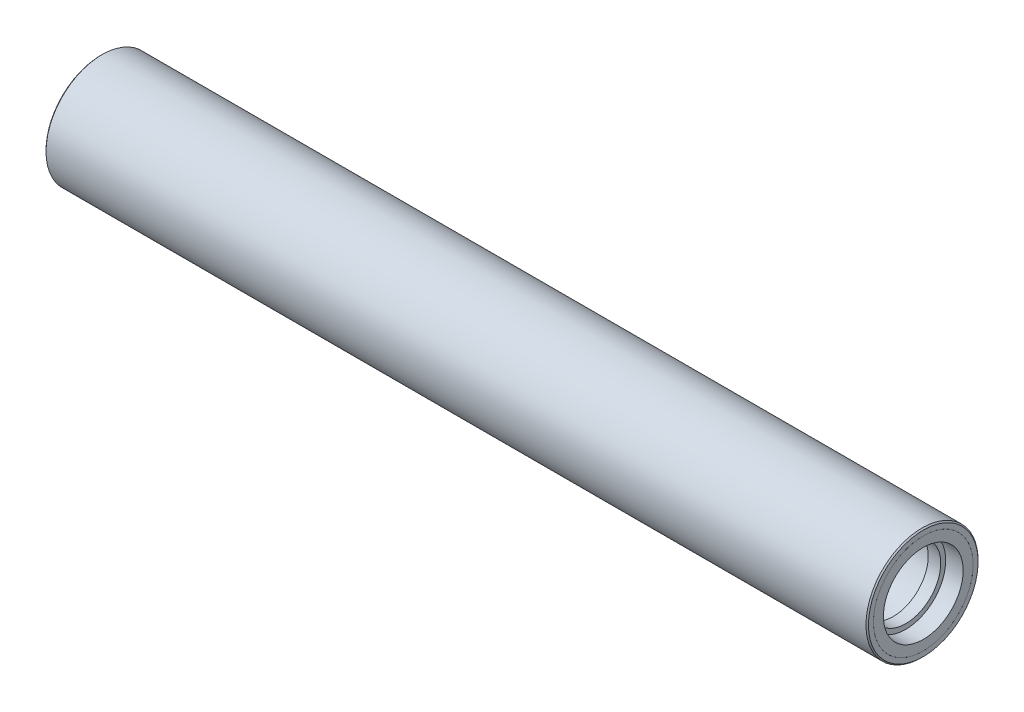
from build123d import *

# Parameters (mm, degrees)
CHAMFER1_SIZE       = 0.5
SKETCH2_R           = 20
SKETCH2_R_2         = 14
BOSS_EXTRUDE1_DEPTH = 12
SKETCH4_R           = 16
CUT_EXTRUDE1_DEPTH  = 7
SKETCH5_R           = 20
SKETCH5_R_2         = 14
BOSS_EXTRUDE2_DEPTH = 12
SKETCH7_R           = 16
CUT_EXTRUDE2_DEPTH  = 7


with BuildPart() as part:
    # Sketch1 → Revolve1 (revolve)
    with BuildSketch(Plane.XY, mode=Mode.PRIVATE) as revolve1_sk:
        Polygon((35.121064285, 17.5), (341.121064285, 17.5), (341.121064285, 20), (353.121064285, 20), (353.121064285, 22.5), (23.121064285, 22.5), (23.121064285, 20), (35.121064285, 20), align=None)
    revolve(revolve1_sk.sketch.rotate(Axis((0, 0, 0), (1, 0, 0)), 90), axis=Axis((0, 0, 0), (1, 0, 0)))

    # Chamfer1
    chamfer1_edges = [part.edges().sort_by_distance(p)[0] for p in [
        (353.121064285, 0, -22.5),
        (23.121064285, 0, -22.5),
    ]]
    chamfer(chamfer1_edges, length=CHAMFER1_SIZE)


with BuildPart() as body_2:
    # Sketch2 → Boss-Extrude1 (new body)
    with BuildSketch(Plane(origin=(341.121064285, 0, 0), x_dir=(0, 0, -1), z_dir=(1, 0, 0))):
        Circle(SKETCH2_R)
        Circle(SKETCH2_R_2, mode=Mode.SUBTRACT)
    extrude(amount=BOSS_EXTRUDE1_DEPTH)

    # Sketch4 → Cut-Extrude1 (cut)
    with BuildSketch(Plane(origin=(353.121064285, 0, 0), x_dir=(0, 0, -1), z_dir=(1, 0, 0))):
        Circle(SKETCH4_R)
    extrude(amount=-CUT_EXTRUDE1_DEPTH, mode=Mode.SUBTRACT)


with BuildPart() as body_3:
    # Sketch5 → Boss-Extrude2 (new body)
    with BuildSketch(Plane.ZY.offset(-35.121064285)):
        Circle(SKETCH5_R)
        Circle(SKETCH5_R_2, mode=Mode.SUBTRACT)
    extrude(amount=BOSS_EXTRUDE2_DEPTH)

    # Sketch7 → Cut-Extrude2 (cut)
    with BuildSketch(Plane.ZY.offset(-23.121064285)):
        Circle(SKETCH7_R)
    extrude(amount=-CUT_EXTRUDE2_DEPTH, mode=Mode.SUBTRACT)


solid = Compound([part.part, body_2.part, body_3.part])
